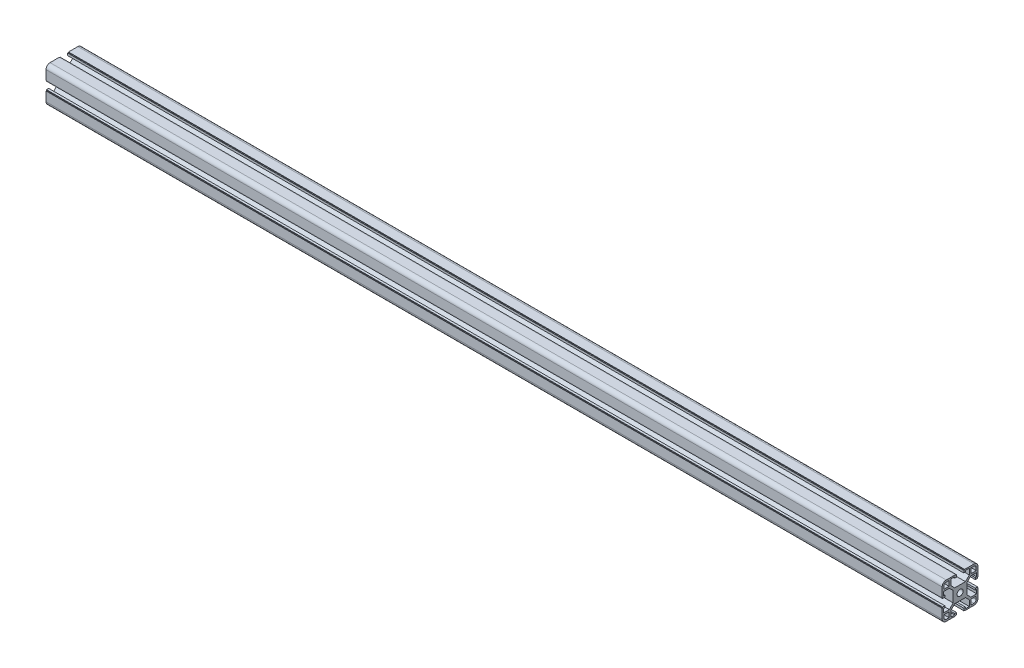
SolidWorks part; units mm, degrees
ref_plane "Front Plane" through (0, 0, 0) normal (0, 0, 1) x (1, 0, 0)
ref_plane "Top Plane" through (0, 0, 0) normal (0, 1, 0) x (1, 0, 0)
ref_plane "Right Plane" through (0, 0, 0) normal (1, 0, 0) x (0, 0, -1)
sketch "草图1" plane through (0, 0, 0) normal (0, 0, 1) x (1, 0, 0)
  line L0 (-484.975, 0) -> (515.025, 0)
  dimension "D1" = 1000
other "Aluminium profile 40 X 40B X R4.5(1)"
ref_plane "Plane1" through (-484.975, 0, 0) normal (1, 0, 0) x (0, 1, 0)
sketch "Sketch1" plane through (-484.975, 0, 0) normal (1, 0, 0) x (0, 1, 0)
  line L0 (-5.1, 20) -> (-5.1, 19.5)
  line L1 (-5.1, 19.5) -> (-4.1, 19.5)
  line L2 (-4.1, 19.5) -> (-4.1, 17)
  line L3 (-6.1, 18.5) -> (-10.3, 18.5)
  line L4 (-15.5, -20) -> (-5.1, -20)
  line L5 (-20, -15.5) -> (-20, -5.1)
  line L6 (15.5, 20) -> (5.1, 20)
  line L7 (20, 15.5) -> (20, 5.1)
  line L8 (0, 14.8756) -> (0, 0) construction
  line L9 (0, 0) -> (14.1675, 0) construction
  line L10 (-10.3, 18.5) -> (-10.3, 12)
  line L11 (-10.3, 12) -> (-6, 7.7)
  line L12 (-6, 7.7) -> (6, 7.7)
  line L13 (10.3, 12) -> (6, 7.7)
  line L14 (10.3, 18.5) -> (10.3, 12)
  line L15 (6.1, 18.5) -> (10.3, 18.5)
  line L16 (4.1, 19.5) -> (4.1, 17)
  line L17 (5.1, 19.5) -> (4.1, 19.5)
  line L18 (5.1, 20) -> (5.1, 19.5)
  line L19 (-5.1, 20) -> (-15.5, 20)
  line L20 (20, 5.1) -> (19.5, 5.1)
  line L21 (12.3, 18) -> (15.5, 18)
  line L22 (12.3, 18) -> (12.3, 12.3)
  line L23 (12.3, 12.3) -> (18, 12.3)
  line L24 (18, 15.5) -> (18, 12.3)
  line L25 (19.5, 5.1) -> (19.5, 4.1)
  line L26 (19.5, 4.1) -> (17, 4.1)
  line L27 (17, 6.1) -> (17, 4.1)
  line L28 (18.5, 6.1) -> (17, 6.1)
  line L29 (18.5, 6.1) -> (18.5, 10.3)
  line L30 (18.5, 10.3) -> (12, 10.3)
  line L31 (12, 10.3) -> (7.7, 6)
  line L32 (7.7, 6) -> (7.7, -6)
  line L33 (12, -10.3) -> (7.7, -6)
  line L34 (18.5, -10.3) -> (12, -10.3)
  line L35 (18.5, -6.1) -> (18.5, -10.3)
  line L36 (18.5, -6.1) -> (17, -6.1)
  line L37 (17, -4.1) -> (17, -6.1)
  line L38 (19.5, -4.1) -> (17, -4.1)
  line L39 (19.5, -5.1) -> (19.5, -4.1)
  line L40 (20, -5.1) -> (19.5, -5.1)
  line L41 (5.1, -20) -> (5.1, -19.5)
  line L42 (5.1, -19.5) -> (4.1, -19.5)
  line L43 (4.1, -19.5) -> (4.1, -17)
  line L44 (6.1, -17) -> (4.1, -17)
  line L45 (6.1, -18.5) -> (6.1, -17)
  line L46 (6.1, -18.5) -> (10.3, -18.5)
  line L47 (10.3, -18.5) -> (10.3, -12)
  line L48 (10.3, -12) -> (6, -7.7)
  line L49 (6, -7.7) -> (-6, -7.7)
  line L50 (-10.3, -12) -> (-6, -7.7)
  line L51 (-10.3, -18.5) -> (-10.3, -12)
  line L52 (-6.1, -18.5) -> (-10.3, -18.5)
  line L53 (-6.1, -18.5) -> (-6.1, -17)
  line L54 (-4.1, -17) -> (-6.1, -17)
  line L55 (-4.1, -19.5) -> (-4.1, -17)
  line L56 (-5.1, -19.5) -> (-4.1, -19.5)
  line L57 (-5.1, -20) -> (-5.1, -19.5)
  line L58 (-20, -5.1) -> (-19.5, -5.1)
  line L59 (5.1, -20) -> (15.5, -20)
  line L60 (-20, 5.1) -> (-20, 15.5)
  line L61 (-19.5, -5.1) -> (-19.5, -4.1)
  line L62 (-6.1, 18.5) -> (-6.1, 17)
  line L63 (-6.1, 17) -> (-4.1, 17)
  line L64 (6.1, 18.5) -> (6.1, 17)
  line L65 (4.1, 17) -> (6.1, 17)
  line L66 (-19.5, -4.1) -> (-17, -4.1)
  line L67 (-15.5, 18) -> (-12.3, 18)
  line L68 (-18, 15.5) -> (-18, 12.3)
  line L69 (-18, 12.3) -> (-12.3, 12.3)
  line L70 (-12.3, 18) -> (-12.3, 12.3)
  line L71 (-17, -6.1) -> (-17, -4.1)
  line L72 (-18.5, -6.1) -> (-17, -6.1)
  line L73 (-18.5, -6.1) -> (-18.5, -10.3)
  line L74 (-18.5, -10.3) -> (-12, -10.3)
  line L75 (-12, -10.3) -> (-7.7, -6)
  line L76 (-7.7, -6) -> (-7.7, 6)
  line L77 (-12, 10.3) -> (-7.7, 6)
  line L78 (-18.5, 10.3) -> (-12, 10.3)
  line L79 (-18.5, 6.1) -> (-18.5, 10.3)
  line L80 (-18.5, 6.1) -> (-17, 6.1)
  line L81 (-17, 4.1) -> (-17, 6.1)
  line L82 (-19.5, 4.1) -> (-17, 4.1)
  line L83 (-19.5, 5.1) -> (-19.5, 4.1)
  line L84 (-20, 5.1) -> (-19.5, 5.1)
  line L85 (20, -5.1) -> (20, -15.5)
  line L87 (-18, -12.3) -> (-12.3, -12.3)
  line L88 (-18, -12.3) -> (-18, -15.5)
  line L89 (-15.5, -18) -> (-12.3, -18)
  line L90 (-12.3, -12.3) -> (-12.3, -18)
  line L91 (12.3, -12.3) -> (18, -12.3)
  line L92 (12.3, -12.3) -> (12.3, -18)
  line L93 (12.3, -18) -> (15.5, -18)
  line L94 (18, -12.3) -> (18, -15.5)
  circle A0 centre (0, 0) radius 3.4
  arc A1 (-20, 15.5) -> (-15.5, 20) centre (-15.5, 15.5) cw
  arc A2 (20, 15.5) -> (15.5, 20) centre (15.5, 15.5) ccw
  arc A3 (-15.5, -20) -> (-20, -15.5) centre (-15.5, -15.5) cw
  arc A4 (15.5, -20) -> (20, -15.5) centre (15.5, -15.5) ccw
  arc A5 (-15.5, 18) -> (-18, 15.5) centre (-15.5, 15.5) ccw
  arc A6 (18, 15.5) -> (15.5, 18) centre (15.5, 15.5) ccw
  arc A7 (18, -15.5) -> (15.5, -18) centre (15.5, -15.5) cw
  arc A8 (-18, -15.5) -> (-15.5, -18) centre (-15.5, -15.5) ccw
  point P2 (0, 10)
  point P4 (0, 0)
  point P5 (-20, -20)
  point P6 (20, -20)
  point P7 (20, 20)
  point P8 (-20, 20)
  point P36 (-20, 20)
  point P39 (20, 20)
  point P121 (0, 0)
  dimension "D1" = 20.6
  dimension "D2" = 40
  dimension "D3" = 8.2
  dimension "D4" = 10.2
  dimension "D5" = 12.3
  dimension "D6" = 6.8
  dimension "D7" = 4.5
  dimension "D8" = 45
  dimension "D12" = 2
  dimension "D13" = 5.7
  dimension "D14" = 2
  dimension "D18" = 2.5
  dimension "D19" = 2.5
  dimension "D15" = 2.5
  dimension "D9" = 0.5
  dimension "D10" = 1.5
  dimension "D11" = 12
  dimension "D16" = 3
  dimension "D17" = 2
  dimension "D20" = 2
  dimension "D21" = 2
